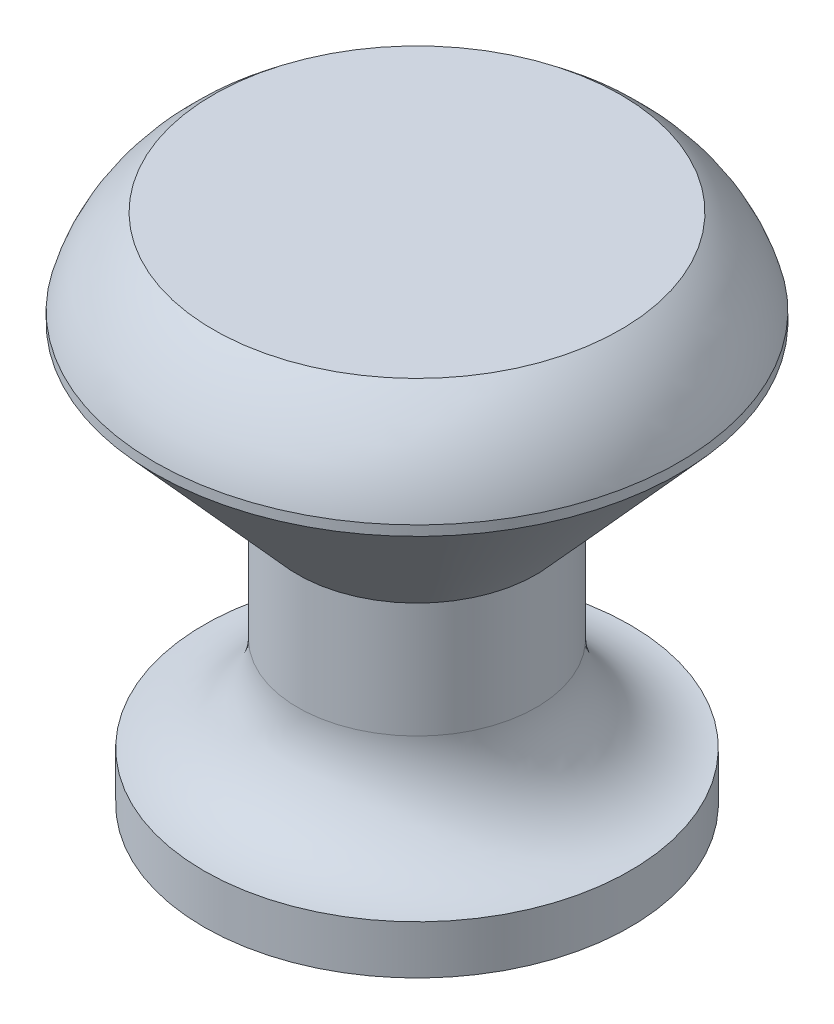
SolidWorks part; units mm, degrees
ref_plane "Front Plane" through (0, 0, 0) normal (0, 0, 1) x (1, 0, 0)
ref_plane "Top Plane" through (0, 0, 0) normal (0, 1, 0) x (1, 0, 0)
ref_plane "Right Plane" through (0, 0, 0) normal (1, 0, 0) x (0, 0, -1)
sketch "Sketch1" plane through (0, 0, 0) normal (1, 0, 0) x (0, 0, -1)
  line L0 (0, 0) -> (10.725, 0)
  line L1 (10.725, 0) -> (10.725, 2.45)
  line L2 (6, 7.2053) -> (6, 0) construction
  line L3 (0, 0) -> (0, 25.8)
  line L4 (6, 13) -> (13.2002, 21)
  line L5 (13.2002, 21) -> (13.2002, 21.5)
  line L6 (0, 0) -> (0, 25.8) construction
  line L7 (0, 25.8) -> (10.25, 25.8)
  line L8 (6, 13) -> (6, 7.2053)
  arc A0 (6, 7.2053) -> (10.725, 2.45) centre (10.7554, 7.2053) ccw
  arc A1 (13.2002, 21.5) -> (10.25, 25.8) centre (5.7285, 19.5357) ccw
  dimension "D9" = 4.7554
  dimension "D11" = 7.7256
  dimension "D1" = 10.725
  dimension "D2" = 2.45
  dimension "D3" = 6
  dimension "D4" = 21
  dimension "D5" = 13
  dimension "D6" = 0.5
  dimension "D7" = 25.8
  dimension "D8" = 10.25
  dimension "D10" = 138.012
revolve "Revolve1" add sketch "Sketch1" angle 360 about L3
hole_wizard "M4 Tapped Hole1" positions "Sketch2" profile "Sketch4" tap size "M4" standard "GB"
sketch "Sketch2" plane through (0, 0, 0) normal (0, -1, 0) x (-1, 0, 0)
  point P0 (0, 0)
sketch "Sketch4" plane through (0, 0, 0) normal (1, 0, 0) x (0, 0, -1)
  line L0 (0, 0) -> (0, 11.0914)
  line L1 (0, 11.0914) -> (1.65, 10.1)
  line L2 (1.65, 10.1) -> (1.65, 0)
  line L5 (1.65, 0) -> (0, 0)
  line L10 (0, 11.0914) -> (-1.65, 10.1) construction
  line L11 (0, -6.35) -> (0, 107.95) construction
  dimension "螺纹孔钻头直径" = 3.3
  dimension "螺纹孔钻头深度" = 10.1
  dimension "导头角度" = 118
cosmetic thread "Cosmetic Thread1" parameters "D1"=8, "D2"=4
